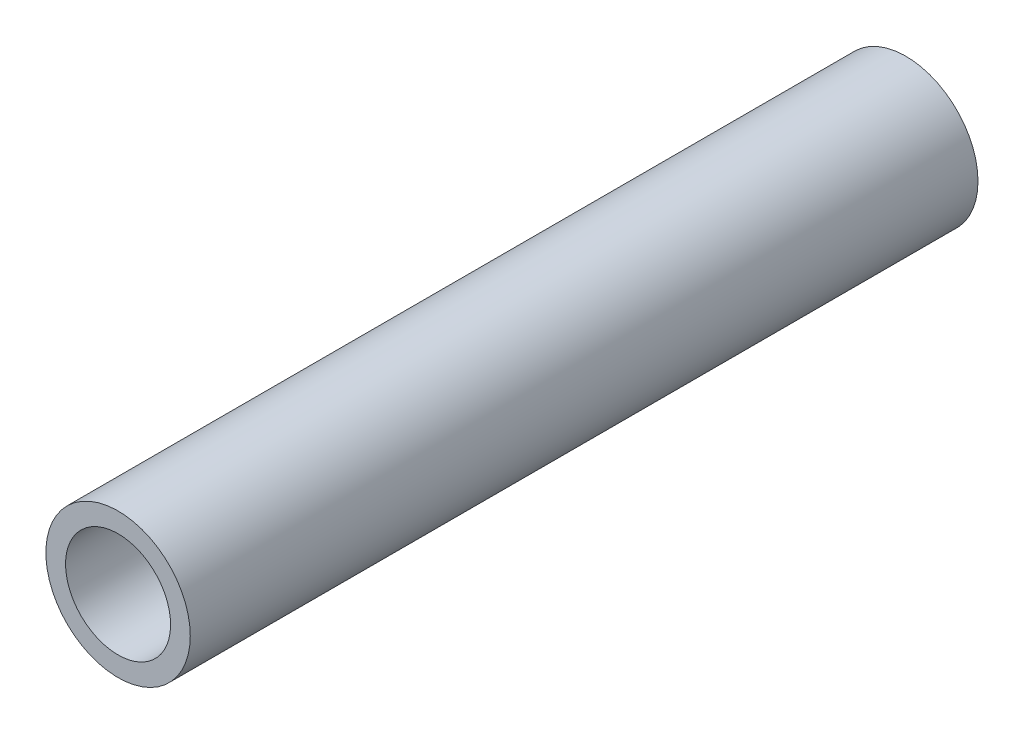
from build123d import *

# Parameters (mm, degrees)
SKETCH_1_R           = 11
SKETCH_1_R_2         = 8
BOSS_EXTRUDE_1_DEPTH = 120


with BuildPart() as part:
    # Sketch 1 → Boss-Extrude 1 (new body)
    with BuildSketch(Plane.XY):
        Circle(SKETCH_1_R)
        Circle(SKETCH_1_R_2, mode=Mode.SUBTRACT)
    extrude(amount=BOSS_EXTRUDE_1_DEPTH)


solid = part.part
